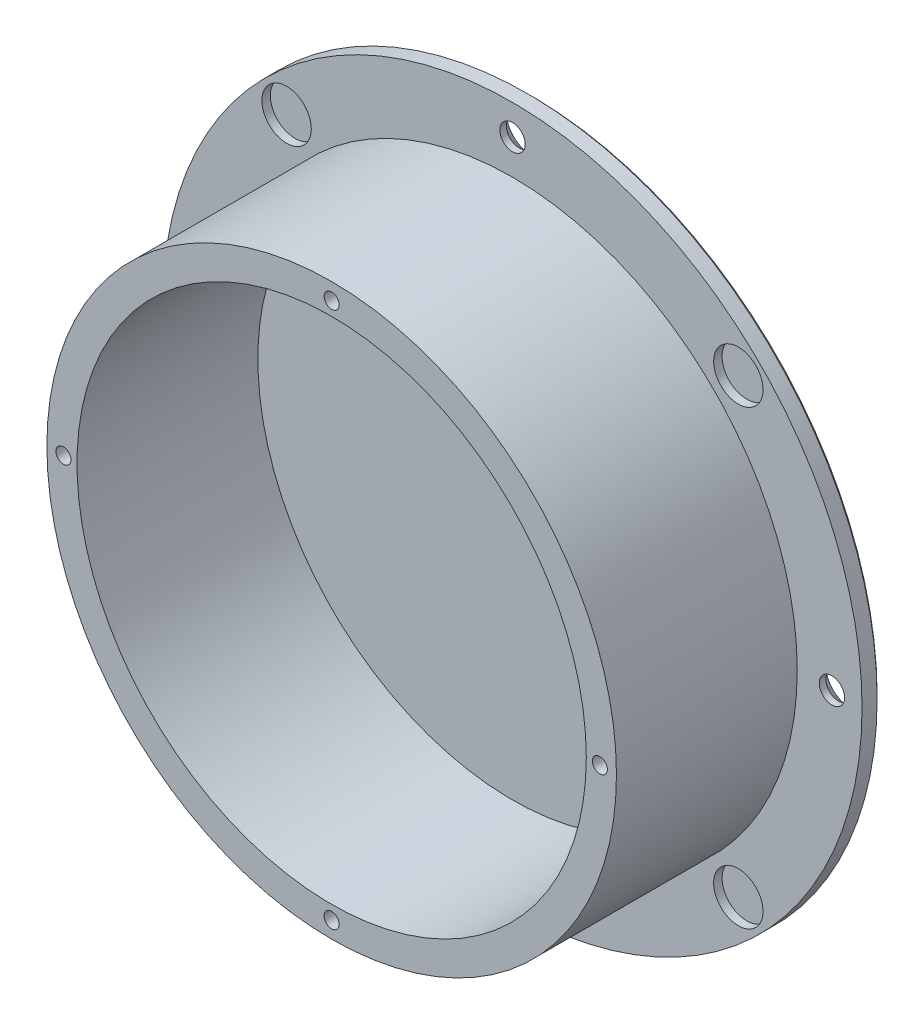
SolidWorks part; units mm, degrees
ref_plane "前视基准面" through (0, 0, 0) normal (0, 0, 1) x (1, 0, 0)
ref_plane "上视基准面" through (0, 0, 0) normal (0, 1, 0) x (1, 0, 0)
ref_plane "右视基准面" through (0, 0, 0) normal (1, 0, 0) x (0, 0, -1)
sketch "草图1" plane through (0, 0, 0) normal (0, 0, 1) x (1, 0, 0)
  circle A0 centre (0, 0) radius 58
  dimension "D1" = 116
extrude "凸台-拉伸1" add sketch "草图1" along normal blind 3
sketch "草图2" plane through (0, 0, 3) normal (0, 0, 1) x (1, 0, 0)
  circle A0 centre (0, 0) radius 47.25
  circle A1 centre (0, 0) radius 42.25
  dimension "D1" = 94.5
  dimension "D2" = 5
extrude "凸台-拉伸2" add sketch "草图2" along normal blind 30
chamfer "倒角1" distance 0.5 angle 45 1 edges at (58, 0, 0)
hole_wizard "M4 六角凹锥坑螺钉的锥形沉头孔1" positions "草图6" profile "草图7" countersink size "M4" standard "ISO"
sketch "草图6" plane through (0, 0, 0) normal (0, 0, -1) x (-1, 0, 0)
  point P0 (0, 53)
  point P9 (53, 0)
  point P10 (0, -53)
  point P11 (-53, 0)
  dimension "D1" = 53
  dimension "D2" = 4
sketch "草图7" plane through (0, 53, 0) normal (1, 0, 0) x (0, 1, 0)
  line L0 (0, 0) -> (0, 11.3618)
  line L1 (0, 11.3618) -> (2.1, 10.1)
  line L2 (2.1, 10.1) -> (2.1, 1.9)
  line L3 (2.1, 1.9) -> (4, 0)
  line L5 (4, 0) -> (0, 0)
  line L6 (-2.1, 1.9) -> (-4, 0) construction
  line L10 (0, 11.3618) -> (-2.1, 10.1) construction
  line L11 (0, -6.35) -> (0, 107.95) construction
  dimension "孔直径" = 4.2
  dimension "孔深度" = 10.1
  dimension "近端锥形沉头孔直径" = 8
  dimension "近端锥形沉头孔角度" = 90
  dimension "导头角度" = 118
hole_wizard "M3 螺纹孔2" positions "草图30" profile "草图31" tap size "M3" standard "GB"
sketch "草图30" plane through (0, 0, 33) normal (0, 0, 1) x (1, 0, 0)
  point P0 (0, 44.5)
  point P9 (44.5, 0)
  point P10 (0, -44.5)
  point P11 (-44.5, 0)
  point P12 (0, 0)
  dimension "D1" = 44.5
  dimension "D2" = 4
sketch "草图31" plane through (0, 44.5, 33) normal (1, 0, 0) x (0, -1, 0)
  line L0 (0, 0) -> (0, 8.2511)
  line L1 (0, 8.2511) -> (1.25, 7.5)
  line L2 (1.25, 7.5) -> (1.25, 0)
  line L5 (1.25, 0) -> (0, 0)
  line L10 (0, 8.2511) -> (-1.25, 7.5) construction
  line L11 (0, -6.35) -> (0, 107.95) construction
  dimension "螺纹孔钻头直径" = 2.5
  dimension "螺纹孔钻头深度" = 7.5
  dimension "导头角度" = 118
cosmetic thread "孔螺蚊线1" parameters "D1"=6, "D2"=3
cosmetic thread "孔螺蚊线2" parameters "D1"=6, "D2"=3
cosmetic thread "孔螺蚊线3" parameters "D1"=6, "D2"=3
cosmetic thread "孔螺蚊线4" parameters "D1"=6, "D2"=3
sketch "草图32" plane through (0, 0, 3) normal (0, 0, 1) x (1, 0, 0)
  line L0 (0, 0) -> (53, 0) construction
  line L1 (0, 0) -> (37.4767, -37.4767) construction
  line L2 (0, 0) -> (0, -16.6742) construction
  circle A0 centre (0, 0) radius 53 construction
  circle A1 centre (37.4767, -37.4767) radius 4.1
  circle A2 centre (37.4767, 37.4767) radius 4.1
  circle A3 centre (-37.4767, 37.4767) radius 4.1
  circle A4 centre (-37.4767, -37.4767) radius 4.1
  dimension "D2" = 8.2
  dimension "D1" = 45
extrude "切除-拉伸12" cut sketch "草图32" against normal blind 1.4
